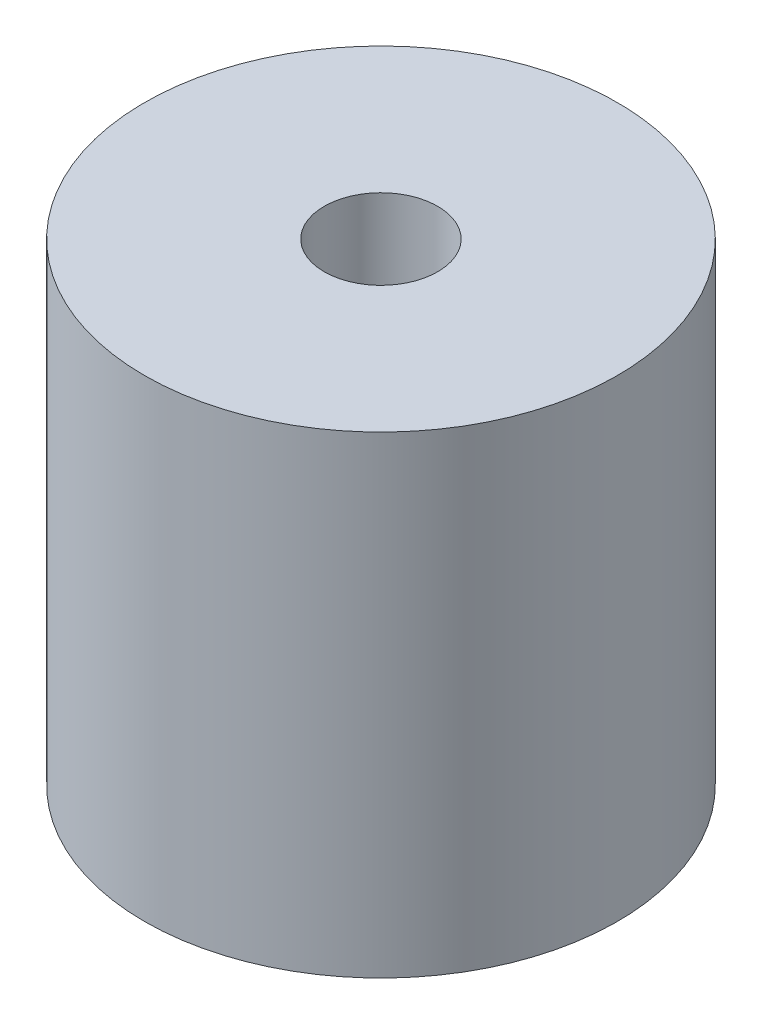
from build123d import *

# Parameters (mm, degrees)
SKETCH1_R           = 12.5
SKETCH1_R_2         = 3
BOSS_EXTRUDE1_DEPTH = 25


with BuildPart() as part:
    # Sketch1 → Boss-Extrude1 (new body)
    with BuildSketch(Plane(origin=(0, 0, 0), x_dir=(1, 0, 0), z_dir=(0, 1, 0))):
        with Locations(Location((0, 0, 0), (0, 0, 270))):
            Circle(SKETCH1_R)
        with Locations(Location((0, 0, 0), (0, 0, 270))):
            Circle(SKETCH1_R_2, mode=Mode.SUBTRACT)
    extrude(amount=BOSS_EXTRUDE1_DEPTH)


solid = part.part
